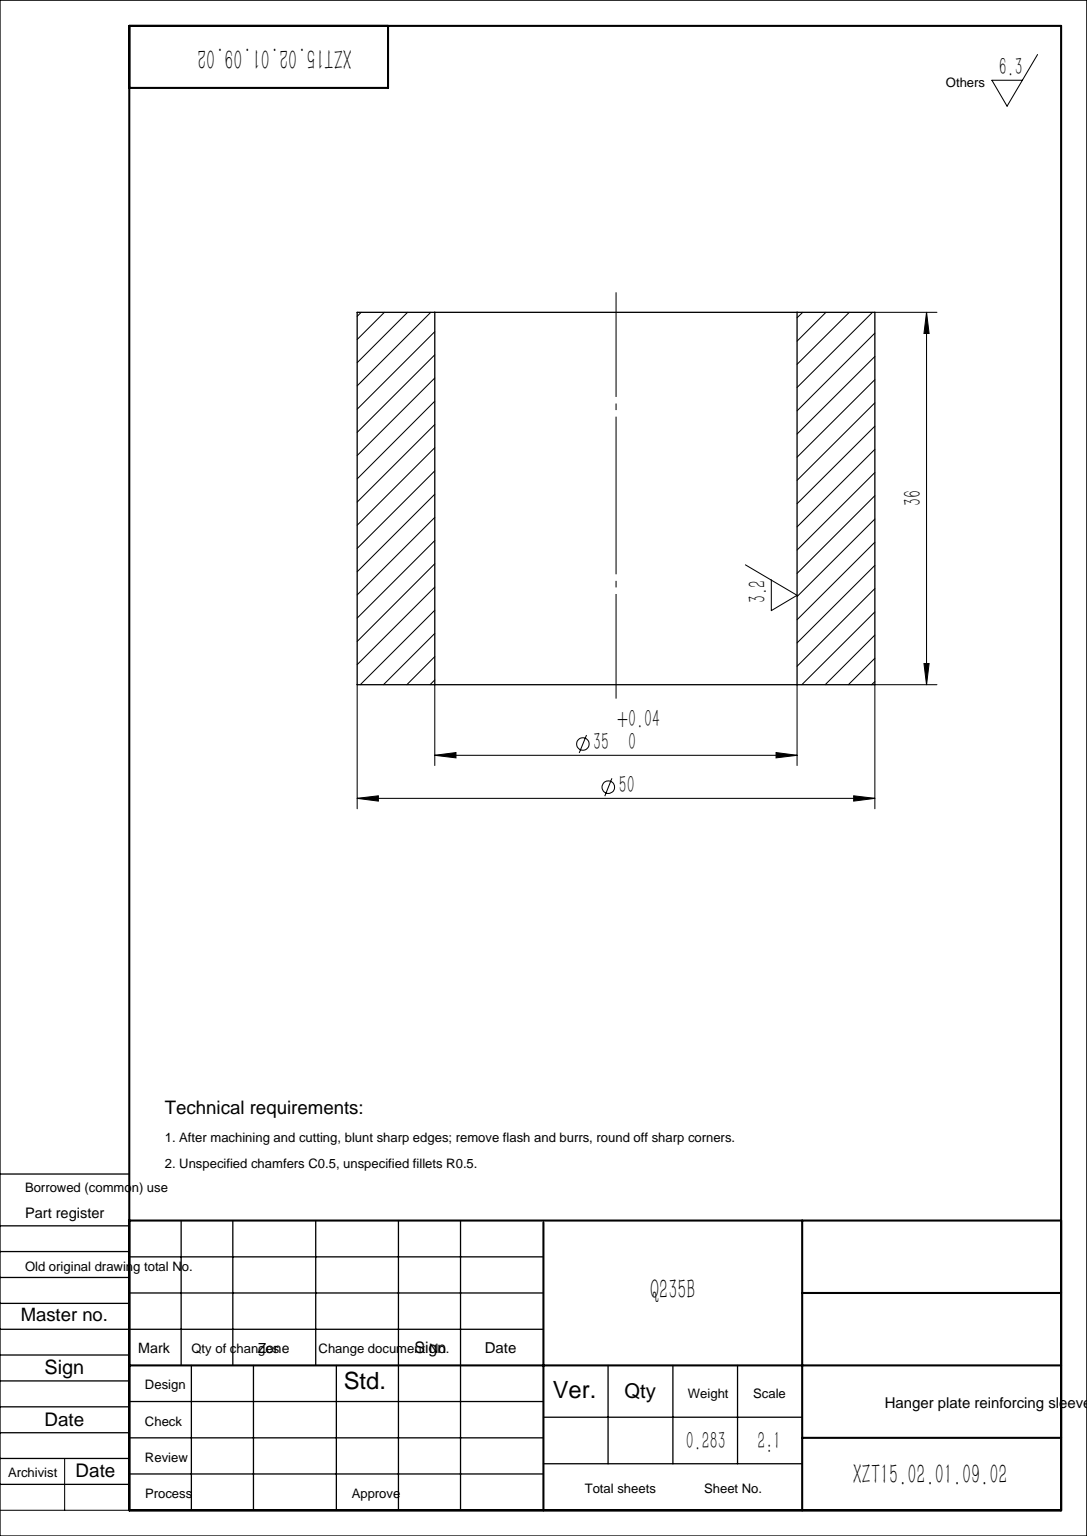
SolidWorks part; units mm, degrees
material "Q235B"
ref_plane "Front Plane" through (0, 0, 0) normal (0, 0, 1) x (1, 0, 0)
ref_plane "Top Plane" through (0, 0, 0) normal (0, 1, 0) x (1, 0, 0)
ref_plane "Right Plane" through (0, 0, 0) normal (1, 0, 0) x (0, 0, -1)
sketch "Sketch1" plane through (0, 0, 0) normal (0, 1, 0) x (1, 0, 0)
  circle A0 centre (0, 0) radius 17.5
  circle A1 centre (0, 0) radius 25
  dimension "D1" = 35
  dimension "D2" = 50
extrude "Boss-Extrude1" add sketch "Sketch1" along normal blind 36
